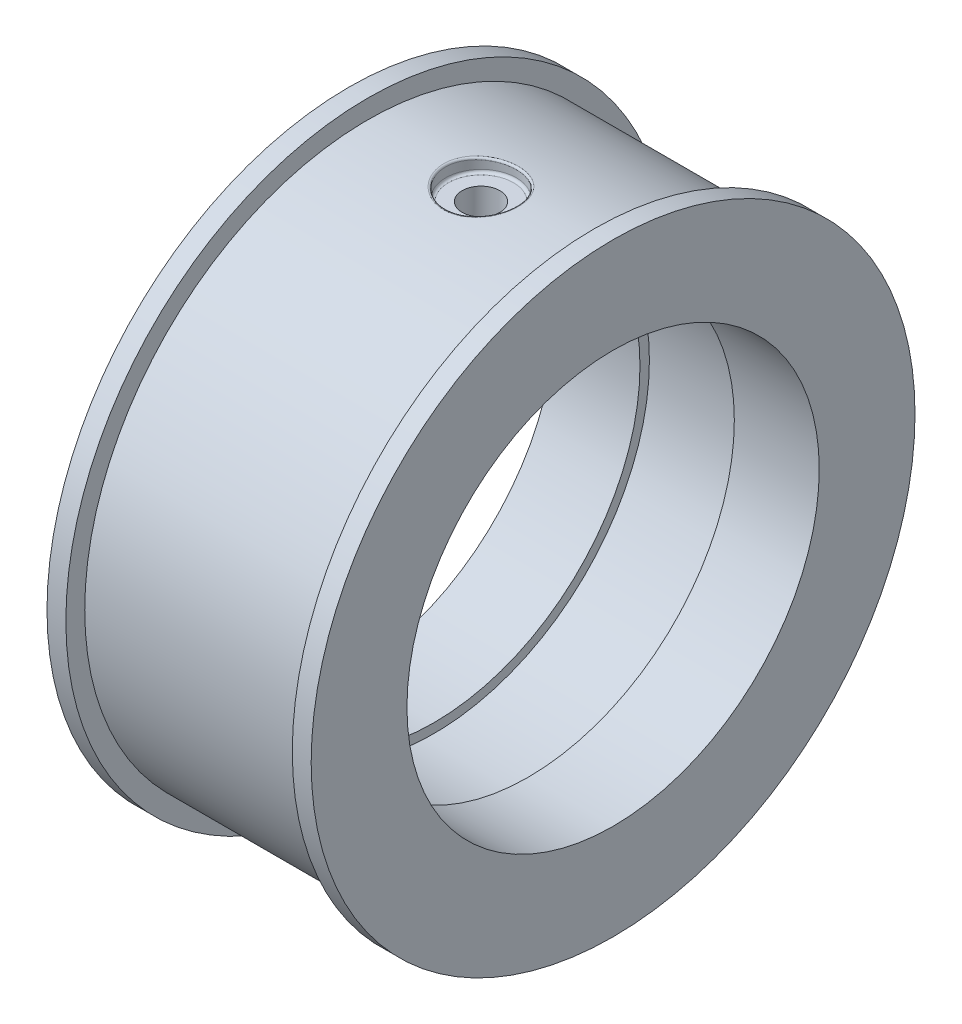
SolidWorks part; units mm, degrees
ref_plane "Front Plane" through (0, 0, 0) normal (0, 0, 1) x (1, 0, 0)
ref_plane "Top Plane" through (0, 0, 0) normal (0, 1, 0) x (1, 0, 0)
ref_plane "Right Plane" through (0, 0, 0) normal (1, 0, 0) x (0, 0, -1)
sketch "Sketch1" plane through (0, 0, 0) normal (0, 0, 1) x (1, 0, 0)
  line L0 (-19.0368, 0) -> (19.2228, 0) construction
  line L1 (-8.3897, 21.85) -> (-8.3897, 32)
  line L2 (-8.3897, 32) -> (-6.3897, 32)
  line L3 (-6.3897, 32) -> (-6.3897, 30)
  line L4 (-6.3897, 30) -> (17.6103, 30)
  line L5 (17.6103, 30) -> (17.6103, 32)
  line L6 (17.6103, 32) -> (19.6103, 32)
  line L7 (19.6103, 32) -> (19.6103, 21.85)
  line L8 (19.6103, 21.85) -> (10.6103, 21.85)
  line L9 (10.6103, 21.85) -> (10.6103, 22.85)
  line L10 (10.6103, 22.85) -> (0.6103, 22.85)
  line L11 (0.6103, 22.85) -> (0.6103, 21.85)
  line L12 (0.6103, 21.85) -> (-8.3897, 21.85)
  dimension "D2" = 28
  dimension "D3" = 24
  dimension "D4" = 2
  dimension "D5" = 21.85
  dimension "D6" = 21.85
  dimension "D7" = 22.85
  dimension "D8" = 10
  dimension "D9" = 9
  dimension "D10" = 30
  dimension "D11" = 32
  dimension "D12" = 32
revolve "Revolve1" add sketch "Sketch1" angle 360 about L0
ref_plane "Plane1" through (0, 30, 0) normal (0, 1, 0) x (1, 0, 0)
sketch "Sketch2" plane through (0, 30, 0) normal (0, 1, 0) x (1, 0, 0)
  line L0 (-6.3897, 0) -> (17.6103, 0)
  line L1 (-6.3897, -32) -> (-6.3897, 32) construction
  line L2 (17.6103, 30) -> (17.6103, -30) construction
hole_wizard "Hole1" positions "Sketch3" profile "Sketch4" legacy
sketch "Sketch3" plane through (0, 30, 0) normal (0, 1, 0) x (1, 0, 0)
  line L0 (-6.3897, 0) -> (17.6103, 0) construction
  point P0 (5.6103, 0)
sketch "Sketch4" plane through (5.6103, 30, 0) normal (1, 0, 0) x (0, 0, 1)
  line L0 (0, 0) -> (0, 1.5)
  line L1 (0, 1.5) -> (3.75, 1.5)
  line L2 (3.75, 1.5) -> (3.75, 0)
  line L3 (3.75, 0) -> (0, 0)
  line L4 (0, 110) -> (0, -10) construction
  dimension "直径" = 7.5
  dimension "深度" = 1.5
hole_wizard "Hole2" positions "Sketch5" profile "Sketch6" legacy
sketch "Sketch5" plane through (0, 28.5, 0) normal (0, 1, 0) x (1, 0, 0)
  point P0 (5.6103, 0)
sketch "Sketch6" plane through (5.6103, 28.5, 0) normal (1, 0, 0) x (0, 0, 1)
  line L0 (0, 0) -> (0, 5.65)
  line L1 (0, 5.65) -> (2, 5.65)
  line L2 (2, 5.65) -> (2, 0)
  line L3 (2, 0) -> (0, 0)
  line L4 (0, 110) -> (0, -10) construction
  dimension "直径" = 4
  dimension "深度" = 5.65
ref_plane "Plane2" through (0, -30, 0) normal (0, -1, 0) x (-1, 0, 0)
sketch "Sketch8" plane through (0, -30, 0) normal (0, -1, 0) x (-1, 0, 0)
  line L0 (6.3897, 0) -> (-17.6103, 0) construction
  line L1 (6.3897, 0) -> (-17.6103, 0)
hole_wizard "Dowel Hole1" positions "Sketch9" profile "Sketch10" hole size "Ø4.0" standard "GB"
sketch "Sketch9" plane through (0, -30, 0) normal (0, -1, 0) x (-1, 0, 0)
  line L0 (6.3897, 0) -> (-17.6103, 0) construction
  point P0 (-5.6103, 0)
sketch "Sketch10" plane through (5.6103, -30, 0) normal (1, 0, 0) x (0, 0, -1)
  line L0 (0, 0) -> (0, 5.2017)
  line L1 (0, 5.2017) -> (2, 4)
  line L2 (2, 4) -> (2, 0)
  line L5 (2, 0) -> (0, 0)
  line L10 (0, 5.2017) -> (-2, 4) construction
  line L11 (0, -6.35) -> (0, 107.95) construction
  dimension "孔直径" = 4
  dimension "孔深度" = 4
  dimension "导头角度" = 118
fillet "Fillet1" radius 0.2 1 edges at (6.44, 29.7763, -3.6571)
fillet "Fillet2" radius 0.3 1 edges at (5.6103, 28.5, 3.75)
